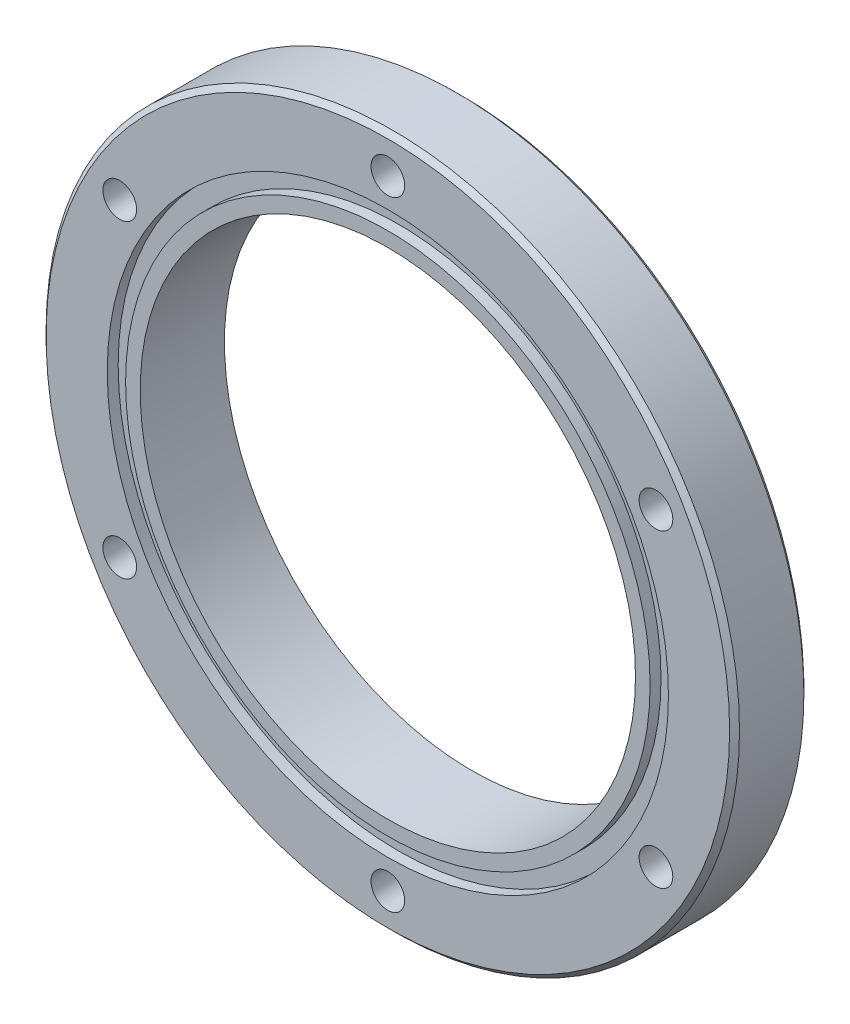
from build123d import *

# Parameters (mm, degrees)
SKETCH1_R             = 70
SKETCH1_R_2           = 50
BOSS_EXTRUDE1_DEPTH   = 17
SKETCH2_R             = 56.65
SKETCH2_R_2           = 52.95
CUT_EXTRUDE1_DEPTH    = 2.2
SKETCH3_R             = 70
SKETCH3_R_2           = 51.5
CUT_EXTRUDE2_DEPTH    = 2
SKETCH4_R             = 3
CUT_EXTRUDE3_DEPTH    = 10
M8_TAPPED_HOLE1_D     = 6.8
M8_TAPPED_HOLE1_DEPTH = 10
M8_TAPPED_HOLE1_TIP   = 2.042926105
CHAMFER1_SIZE         = 1


with BuildPart() as part:
    # Sketch1 → Boss-Extrude1 (new body)
    with BuildSketch(Plane.XY):
        Circle(SKETCH1_R)
        Circle(SKETCH1_R_2, mode=Mode.SUBTRACT)
    extrude(amount=BOSS_EXTRUDE1_DEPTH)

    # Sketch2 → Cut-Extrude1 (cut)
    with BuildSketch(Plane.XY.offset(17)):
        Circle(SKETCH2_R)
        Circle(SKETCH2_R_2, mode=Mode.SUBTRACT)
    extrude(amount=-CUT_EXTRUDE1_DEPTH, mode=Mode.SUBTRACT)

    # Sketch3 → Cut-Extrude2 (cut)
    with BuildSketch(Plane(origin=(0, 0, 0), x_dir=(-1, 0, 0), z_dir=(0, 0, -1))):
        Circle(SKETCH3_R)
        Circle(SKETCH3_R_2, mode=Mode.SUBTRACT)
    extrude(amount=-CUT_EXTRUDE2_DEPTH, mode=Mode.SUBTRACT)

    # Sketch4 → Cut-Extrude3 (cut)
    with BuildSketch(Plane.XY.offset(17)):
        with Locations((0, 62.5)):
            Circle(SKETCH4_R)
        with Locations((54.126587737, 31.25)):
            Circle(SKETCH4_R)
        with Locations((54.126587737, -31.25)):
            Circle(SKETCH4_R)
        with Locations((0, -62.5)):
            Circle(SKETCH4_R)
        with Locations((-54.126587737, -31.25)):
            Circle(SKETCH4_R)
        with Locations((-54.126587737, 31.25)):
            Circle(SKETCH4_R)
    extrude(amount=-CUT_EXTRUDE3_DEPTH, mode=Mode.SUBTRACT)

    # M8 Tapped Hole1
    with Locations(Plane.XY.offset(17)):
        with Locations((0, 62.5), (54.126587737, 31.25), (54.126587737, -31.25), (0, -62.5), (-54.126587737, -31.25), (-54.126587737, 31.25)):
            Hole(M8_TAPPED_HOLE1_D / 2, depth=M8_TAPPED_HOLE1_DEPTH)
            with Locations((0, 0, -(M8_TAPPED_HOLE1_DEPTH + M8_TAPPED_HOLE1_TIP / 2))):  # 118° drill point
                Cone(0, M8_TAPPED_HOLE1_D / 2, M8_TAPPED_HOLE1_TIP, mode=Mode.SUBTRACT)

    # Chamfer1
    chamfer1_edges = [part.edges().sort_by_distance(p)[0] for p in [
        (-70, 0, 2),
        (-70, 0, 17),
    ]]
    chamfer(chamfer1_edges, length=CHAMFER1_SIZE)


solid = part.part
